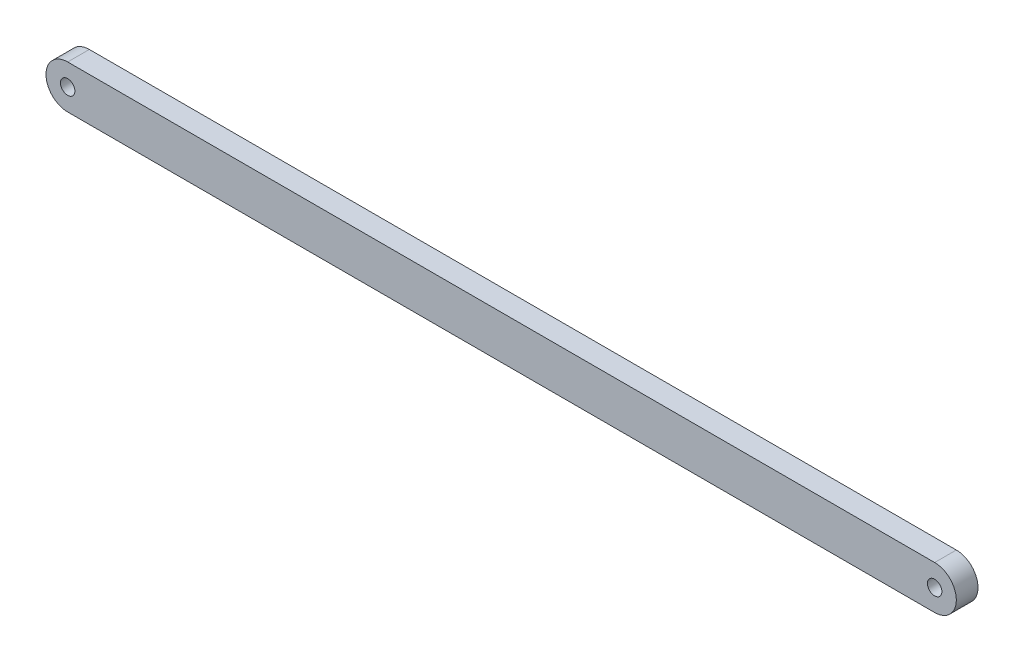
SolidWorks part; units mm, degrees
ref_plane "前视基准面" through (0, 0, 0) normal (0, 0, 1) x (1, 0, 0)
ref_plane "上视基准面" through (0, 0, 0) normal (0, 1, 0) x (1, 0, 0)
ref_plane "右视基准面" through (0, 0, 0) normal (1, 0, 0) x (0, 0, -1)
other "Configuration Table"
sketch "草图1" plane through (0, 0, 0) normal (0, 0, 1) x (1, 0, 0)
  line L0 (-119.7353, 7.1913) -> (120.2647, 7.1913)
  line L1 (-119.7353, -4.8087) -> (120.2647, -4.8087)
  arc A0 (-119.7353, 7.1913) -> (-119.7353, -4.8087) centre (-119.7353, 1.1913) ccw
  arc A1 (120.2647, -4.8087) -> (120.2647, 7.1913) centre (120.2647, 1.1913) ccw
  circle A2 centre (-119.7353, 1.1913) radius 2
  circle A3 centre (120.2647, 1.1913) radius 2
  dimension "D1" = 4
  dimension "D2" = 4
  dimension "D3" = 6
  dimension "D4" = 6
  dimension "D5" = 240
extrude "凸台-拉伸1" add sketch "草图1" along normal blind 6
